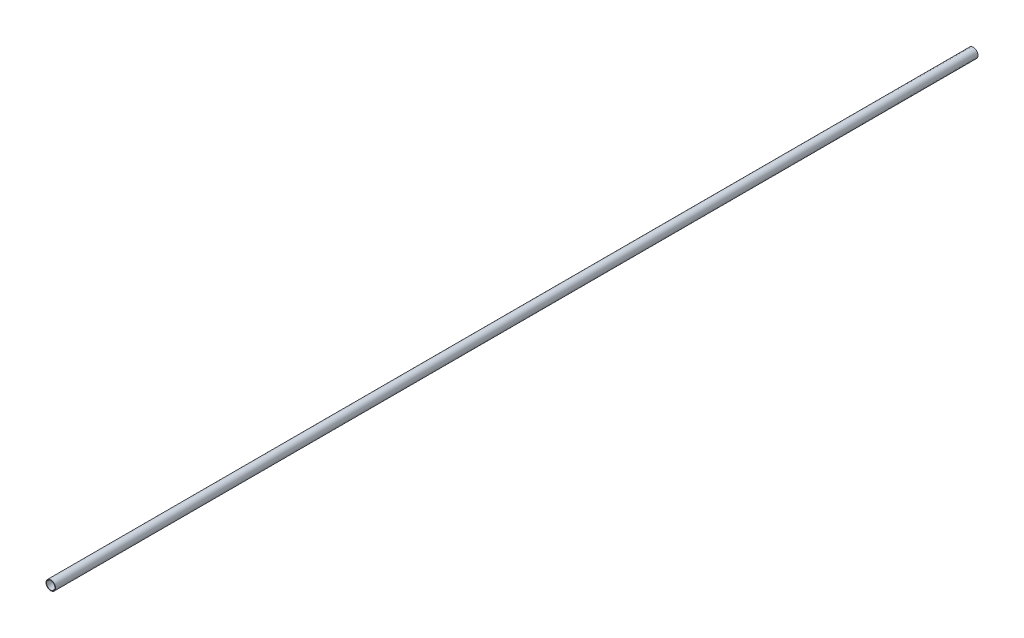
SolidWorks part; units mm, degrees
ref_plane "前视基准面" through (0, 0, 0) normal (0, 0, 1) x (1, 0, 0)
ref_plane "上视基准面" through (0, 0, 0) normal (0, 1, 0) x (1, 0, 0)
ref_plane "右视基准面" through (0, 0, 0) normal (1, 0, 0) x (0, 0, -1)
sketch "草图1" plane through (0, 0, 0) normal (0, 0, 1) x (1, 0, 0)
  circle A0 centre (0, 0) radius 16
  circle A1 centre (0, 0) radius 14
  dimension "D1" = 32
  dimension "D2" = 2
extrude "凸台-拉伸1" add sketch "草图1" along normal mid plane 3100
